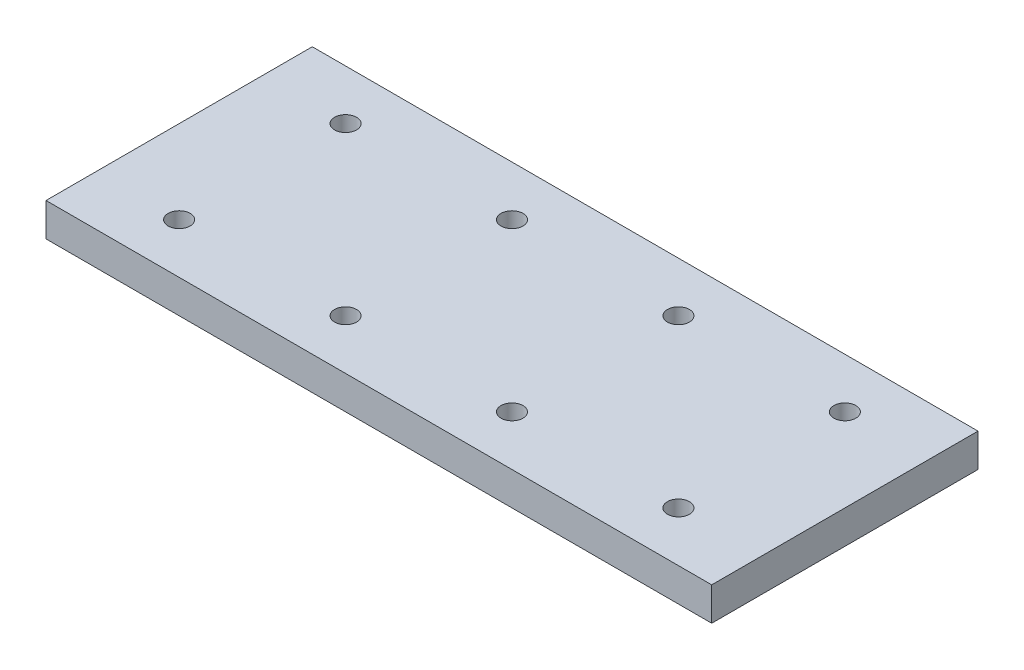
SolidWorks part; units mm, degrees
ref_plane "Front Plane" through (0, 0, 0) normal (0, 0, 1) x (1, 0, 0)
ref_plane "Top Plane" through (0, 0, 0) normal (0, 1, 0) x (1, 0, 0)
ref_plane "Right Plane" through (0, 0, 0) normal (1, 0, 0) x (0, 0, -1)
sketch "Sketch1" plane through (0, 0, 0) normal (0, 1, 0) x (1, 0, 0)
  line L1 (-100, 40) -> (100, 40)
  line L2 (-100, 40) -> (-100, -40)
  line L3 (-100, -40) -> (100, -40)
  line L4 (100, 40) -> (100, -40)
  line L5 (-100, 40) -> (100, -40) construction
  line L6 (-100, -40) -> (100, 40) construction
  point P0 (0, 0)
  dimension "D1" = 80
  dimension "D2" = 200
extrude "Boss-Extrude1" add sketch "Sketch1" along normal blind 10
sketch "Sketch2" plane through (0, 10, 0) normal (0, 1, 0) x (1, 0, 0)
  line L1 (-25, 25) -> (25, 25) construction
  line L2 (-25, 25) -> (-25, -25) construction
  line L3 (-25, -25) -> (25, -25) construction
  line L4 (25, 25) -> (25, -25) construction
  line L5 (-25, 25) -> (25, -25) construction
  line L6 (-25, -25) -> (25, 25) construction
  line L7 (-75, 25) -> (75, 25) construction
  line L8 (-75, 25) -> (-75, -25) construction
  line L9 (-75, -25) -> (75, -25) construction
  line L10 (75, 25) -> (75, -25) construction
  line L11 (-75, 25) -> (75, -25) construction
  line L12 (-75, -25) -> (75, 25) construction
  point P0 (0, 0)
  point P6 (0, 0)
  dimension "D1" = 50
  dimension "D2" = 50
  dimension "D3" = 150
  dimension "D4" = 50
hole_wizard "Ø6.6 (6.6) Diameter Hole1" positions "Sketch3" profile "Sketch4" hole size "Ø6.6" standard "GB" end condition up to next
sketch "Sketch3" plane through (0, 10, 0) normal (0, 1, 0) x (1, 0, 0)
  point P0 (-25, 25)
  point P3 (25, 25)
  point P6 (-25, -25)
  point P9 (25, -25)
  point P12 (-75, 25)
  point P15 (75, 25)
  point P18 (75, -25)
  point P21 (-75, -25)
sketch "Sketch4" plane through (-25, 10, -25) normal (1, 0, 0) x (0, 0, 1)
  line L0 (0, 0) -> (0, 10)
  line L1 (0, 10) -> (3.3, 10)
  line L2 (3.3, 10) -> (3.3, 0)
  line L5 (3.3, 0) -> (0, 0)
  line L11 (0, -6.35) -> (0, 107.95) construction
  dimension "通孔孔直径" = 6.6
  dimension "通孔孔深度" = 10
